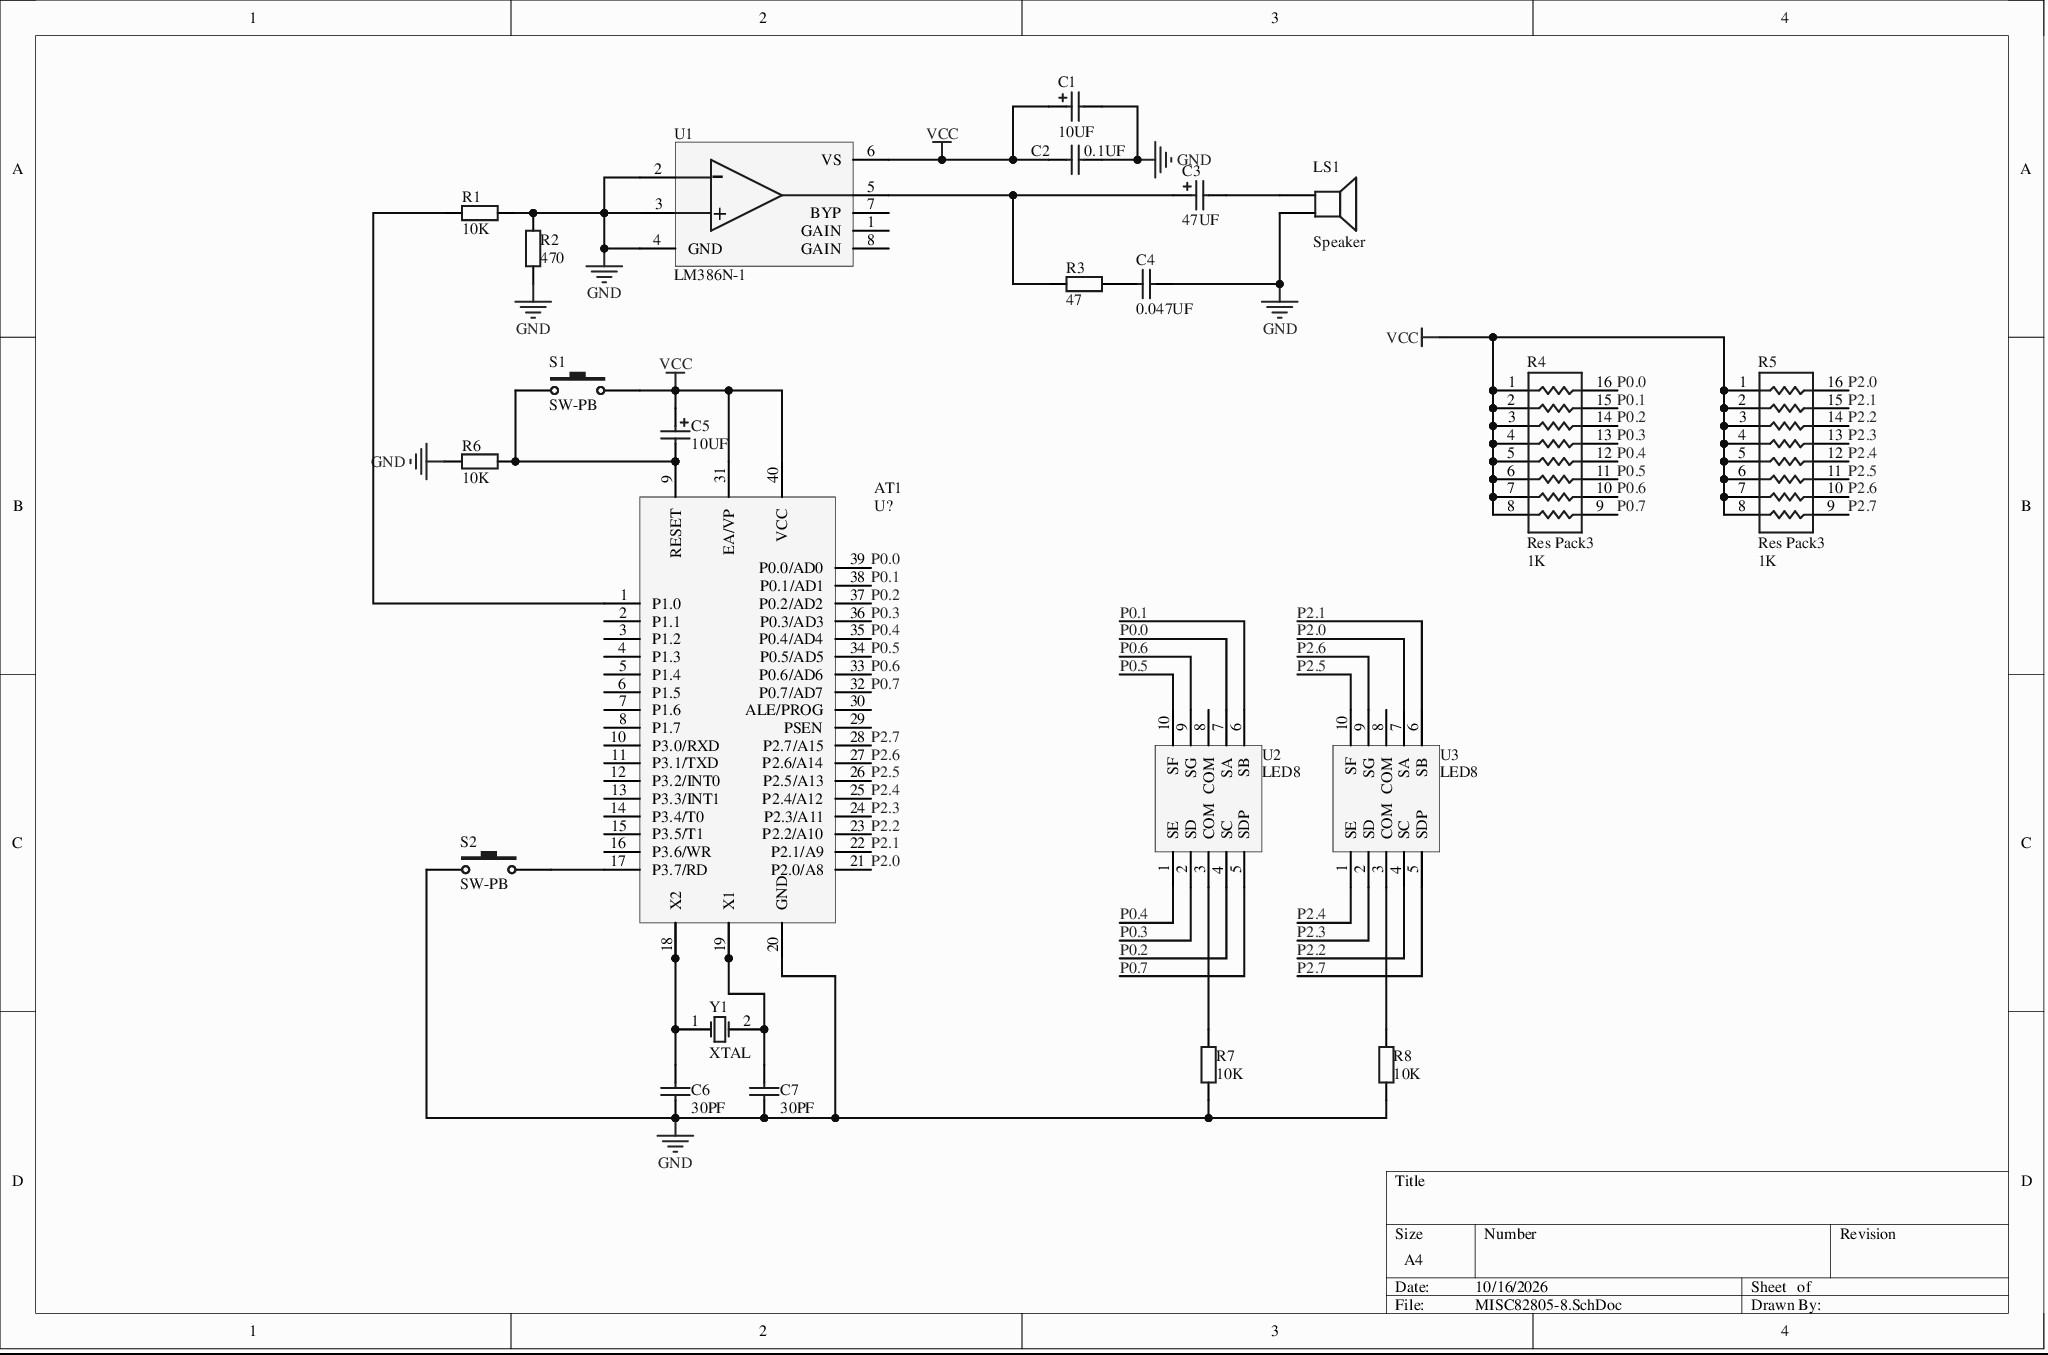
[diagram p0: MISC82805-8.SchDoc]
# Altium project MISC82805-2.PrjPcb
1 sheet, 23 parts. Net scope: global (net labels, ports and power ports of the same name join across sheets).
Board file: MISC82805.PcbDoc

## Sheet MISC82805-8.SchDoc
size A4

### Parts
AT1  U?  [AT89S52]
C1  10UF  [POLAR0.8]
C2  0.1UF  [RAD-0.3]
C3  47UF  [POLAR0.8]
C4  0.047UF  [RAD-0.3]
C5  10UF  [POLAR0.8]
C6  30PF  [RAD-0.3]
C7  30PF  [RAD-0.3]
LS1  Speaker  [PIN2]
R1  10K  [AXIAL-0.4]
R2  470  [AXIAL-0.4]
R3  47  [AXIAL-0.4]
R4  Res Pack3  value 1K  [SO-16_N]
R5  Res Pack3  value 1K  [SO-16_N]
R6  10K  [AXIAL-0.4]
R7  10K  [AXIAL-0.4]
R8  10K  [AXIAL-0.4]
S1  SW-PB  [SPST-2]
S2  SW-PB  [SPST-2]
U1  LM386N-1  [LM386N-1]
U2  LED8  [LED8]
U3  LED8  [LED8]
Y1  XTAL  [R38]

### Nets
GND: AT1.20(GND) C1.2 C2.2 C4.2 C6.1 C7.1 LS1.2 R1.1 R2.1 R2.2 R6.2 R7.2 R8.2 S2.1 U1.2(GAIN) U1.3(GAIN) U1.4(GND)
VCC: AT1.31(EA/VP) AT1.40(VCC) C1.1 C2.1 C5.1 R4.1 R4.2 R4.3 R4.4 R4.5 R4.6 R4.7 R4.8 R5.1 R5.2 R5.3 R5.4 R5.5 R5.6 R5.7 R5.8 S1.2 U1.6(VS)
P0.0: AT1.39(P0.0/AD0) R4.16 U2.7(SA)
P0.1: AT1.38(P0.1/AD1) R4.15 U2.6(SB)
P0.2: AT1.37(P0.2/AD2) R4.14 U2.4(SC)
P0.3: AT1.36(P0.3/AD3) R4.13 U2.2(SD)
P0.4: AT1.35(P0.4/AD4) R4.12 U2.1(SE)
P0.5: AT1.34(P0.5/AD5) R4.11 U2.10(SF)
P0.6: AT1.33(P0.6/AD6) R4.10 U2.9(SG)
P0.7: AT1.32(P0.7/AD7) R4.9 U2.5(SDP)
P2.0: AT1.21(P2.0/A8) R5.16 U3.7(SA)
P2.1: AT1.22(P2.1/A9) R5.15 U3.6(SB)
P2.2: AT1.23(P2.2/A10) R5.14 U3.4(SC)
P2.3: AT1.24(P2.3/A11) R5.13 U3.2(SD)
P2.4: AT1.25(P2.4/A12) R5.12 U3.1(SE)
P2.5: AT1.26(P2.5/A13) R5.11 U3.10(SF)
P2.6: AT1.27(P2.6/A14) R5.10 U3.9(SG)
P2.7: AT1.28(P2.7/A15) R5.9 U3.5(SDP)
NetAT1_1: AT1.1(P1.0) R1.2
NetAT1_9: AT1.9(RESET) C5.2 R6.1 S1.1
NetAT1_17: AT1.17(P3.7/RD) S2.2
NetAT1_18: AT1.18(X2) C6.2 Y1.1(OSC1)
NetAT1_19: AT1.19(X1) C7.2 Y1.2(OSC2)
NetC3_1: C3.1 R3.1 U1.5(GND)
NetC3_2: C3.2 LS1.1
NetC4_1: C4.1 R3.2
NetR7_1: R7.1 U2.3(COM)
NetR8_1: R8.1 U3.3(COM)

Not connected (* = marked no-connect by the designer): AT1 2(P1.1) 3(P1.2) 4(P1.3) 5(P1.4) 6(P1.5) 7(P1.6) 8(P1.7) 10(P3.0/RXD) 11(P3.1/TXD) 12(P3.2/INT0) 13(P3.3/INT1) 14(P3.4/T0) 15(P3.5/T1) 16(P3.6/WR) 29(PSEN) 30(ALE/PROG); U1 1(GAIN) 7(BYP) 8(GAIN); U2 8(COM); U3 8(COM)

### Library data of the parts
AT1 = AT89S52
C1 C3 C5 = Cap Pol2: Polarized Capacitor (Axial); Value: 100pF; Published: 8-Jun-2000; LatestRevisionDate: 17-Jul-2002; LatestRevisionNote: Re-released for DXP Platform.; PackageReference: POLAR0.8; PackageDescription: Polarized Capacitor; 2 Leads; Publisher: Altium Limited
C2 C4 C6 C7 = Cap: Capacitor; Value: 100pF; Published: 8-Jun-2000; LatestRevisionDate: 17-Jul-2002; LatestRevisionNote: Re-released for DXP Platform.; PackageReference: RAD-0.3; PackageDescription: Radial Cap, Thru-Hole; 2 Leads; 0.3 in Pin Spacing; Publisher: Altium Limited
LS1 = Speaker: Loudspeaker; Published: 24-Mar-1999; LatestRevisionDate: 17-Jul-2002; LatestRevisionNote: Re-released for DXP Platform.; PackageReference: PIN2; Publisher: Altium Limited
R1-R3 R6-R8 = Res2: Resistor; Value: 1K; Published: 8-Jun-2000; LatestRevisionDate: 17-Jul-2002; LatestRevisionNote: Re-released for DXP Platform.; PackageReference: AXIAL-0.4; PackageDescription: Axial Device, Thru-Hole; 2 Leads; 0.4 in Pin Spacing; Publisher: Altium Limited
R4 R5 = Res Pack3: Isolated Resistor Network; Published: 24-Mar-1999; LatestRevisionDate: 29-May-2009; LatestRevisionNote: IPC-7351 Footprint Added.; PackageReference: SO-16; PackageDescription: 16-Pin Small Outline Integrated Circuit 1.27 mm Pitch; Code_JEDEC: MS-012-AC; Code_IPC: SOIC127P600-16; Publisher: Altium Limited
S1 S2 = SW-PB: Switch; Published: 24-Mar-1999; LatestRevisionDate: 17-Jul-2002; LatestRevisionNote: Re-released for DXP Platform.; PackageReference: SPST-2; PackageDescription: Switch; 2 Leads; Publisher: Altium Limited
Y1 = XTAL: Crystal Oscillator; Published: 8-Jun-2000; LatestRevisionDate: 17-Jul-2002; LatestRevisionNote: Re-released for DXP Platform.; PackageReference: R38; PackageDescription: Crystal, Thru-Hole; 2 Leads; Body 3.1 x 8.2 mm (Dia.xH); Publisher: Altium Limited